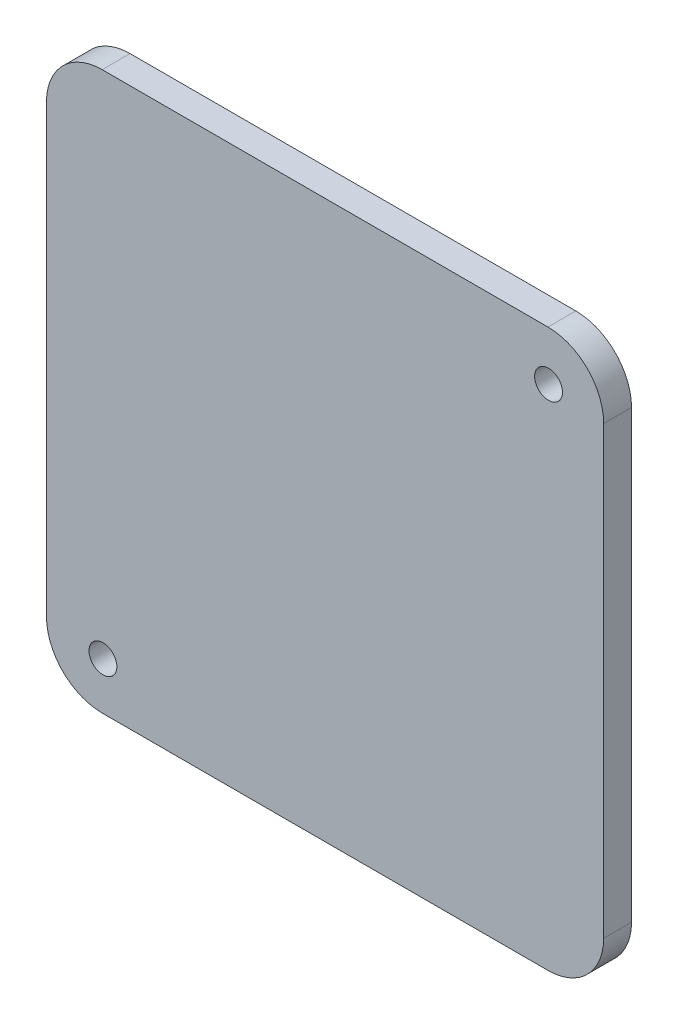
from build123d import *

# Parameters (mm, degrees)
SKETCH1_W           = 20
SKETCH1_H           = 20
BOSS_EXTRUDE1_DEPTH = 1
SKETCH2_R           = 0.5
CUT_EXTRUDE1_DEPTH  = 15.177446879
FILLET1_R           = 2


with BuildPart() as part:
    # Sketch1 → Boss-Extrude1 (new body)
    with BuildSketch(Plane.XY):
        Rectangle(SKETCH1_W, SKETCH1_H)
    extrude(amount=BOSS_EXTRUDE1_DEPTH)

    # Sketch2 → Cut-Extrude1 (cut, through all)
    with BuildSketch(Plane.XY.offset(1)):
        with Locations((-7.973287509, -8.297417088)):
            Circle(SKETCH2_R)
        with Locations((8.021405324, 8.230432172)):
            Circle(SKETCH2_R)
    extrude(amount=-CUT_EXTRUDE1_DEPTH, mode=Mode.SUBTRACT)

    # Fillet1
    fillet1_edges = [part.edges().sort_by_distance(p)[0] for p in [
        (10, -10, 0.5),
        (-10, -10, 0.5),
        (-10, 10, 0.5),
        (10, 10, 0.5),
    ]]
    fillet(fillet1_edges, radius=FILLET1_R)


solid = part.part
